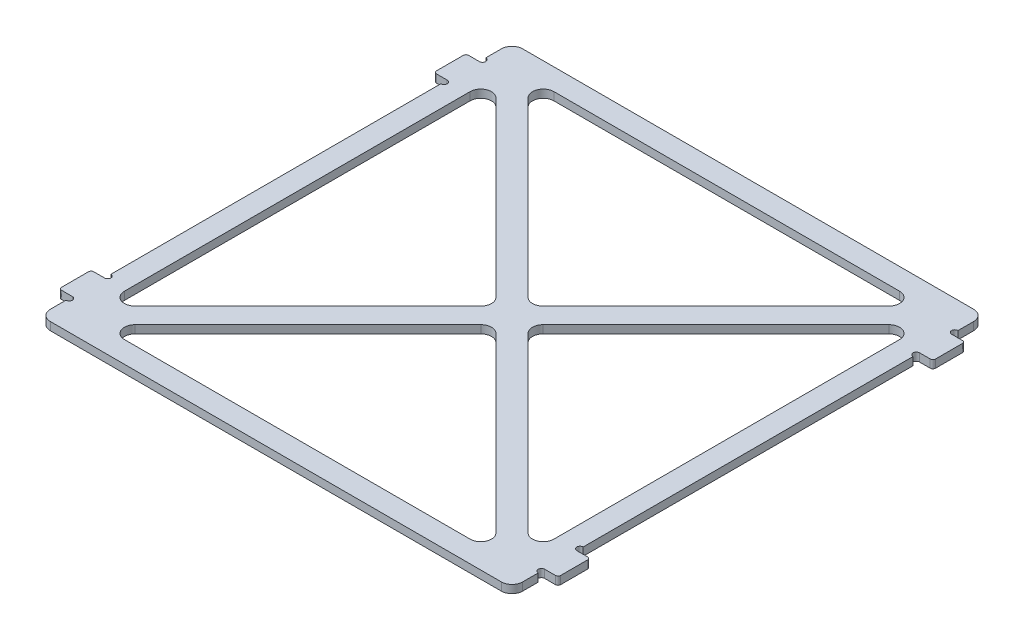
from build123d import *

# Parameters (mm, degrees)
EXTRUDE_1_DEPTH = 1.5
FILLET_1_R      = 0.5
FILLET_2_R      = 2


with BuildPart() as part:
    # 草图1 → 凸台-拉伸1 (new body)
    with BuildSketch(Plane(origin=(0, 0, 0), x_dir=(1, 0, 0), z_dir=(0, 1, 0))):
        with BuildLine():
            Line((44.1, 44.1), (-44.1, 44.1))
            Line((-44.1, 44.1), (-44.1, 39.2))
            ThreePointArc((-44.1, 39.2), (-43.5, 38.6), (-44.1, 38))
            Line((-44.1, 38), (-46.6, 38))
            Line((-46.6, 38), (-46.6, 32))
            Line((-46.6, 32), (-44.1, 32))
            ThreePointArc((-44.1, 32), (-43.5, 31.4), (-44.1, 30.8))
            Line((-44.1, 30.8), (-44.1, -30.8))
            ThreePointArc((-44.1, -30.8), (-43.5, -31.4), (-44.1, -32))
            Line((-44.1, -32), (-46.6, -32))
            Line((-46.6, -32), (-46.6, -38))
            Line((-46.6, -38), (-44.1, -38))
            ThreePointArc((-44.1, -38), (-43.5, -38.6), (-44.1, -39.2))
            Line((-44.1, -39.2), (-44.1, -44.1))
            Line((-44.1, -44.1), (44.1, -44.1))
            Line((44.1, -44.1), (44.1, -39.2))
            ThreePointArc((44.1, -39.2), (43.5, -38.6), (44.1, -38))
            Line((44.1, -38), (46.6, -38))
            Line((46.6, -38), (46.6, -32))
            Line((46.6, -32), (44.1, -32))
            ThreePointArc((44.1, -32), (43.5, -31.4), (44.1, -30.8))
            Line((44.1, -30.8), (44.1, 30.8))
            ThreePointArc((44.1, 30.8), (43.5, 31.4), (44.1, 32))
            Line((44.1, 32), (46.6, 32))
            Line((46.6, 32), (46.6, 38))
            Line((46.6, 38), (44.1, 38))
            ThreePointArc((44.1, 38), (43.5, 38.6), (44.1, 39.2))
            Line((44.1, 39.2), (44.1, 44.1))
        make_face()
        Polygon((-37.1, 40.1), (37.1, 40.1), (0, 3), align=None, mode=Mode.SUBTRACT)
        Polygon((40.1, 37.1), (40.1, -37.1), (3, 0), align=None, mode=Mode.SUBTRACT)
        Polygon((37.1, -40.1), (-37.1, -40.1), (0, -3), align=None, mode=Mode.SUBTRACT)
        Polygon((-40.1, -37.1), (-40.1, 37.1), (-3, 0), align=None, mode=Mode.SUBTRACT)
    extrude(amount=EXTRUDE_1_DEPTH)

    # 圆角1
    fillet_1_edges = [part.edges().sort_by_distance(p)[0] for p in [
        (46.6, 0.75, -38),
        (46.6, 0.75, -32),
        (46.6, 0.75, 32),
        (46.6, 0.75, 38),
        (-46.6, 0.75, 38),
        (-46.6, 0.75, 32),
        (-46.6, 0.75, -32),
        (-46.6, 0.75, -38),
    ]]
    fillet(fillet_1_edges, radius=FILLET_1_R)

    # 圆角2
    fillet_2_edges = [part.edges().sort_by_distance(p)[0] for p in [
        (-44.1, 0.75, -44.1),
        (44.1, 0.75, -44.1),
        (44.1, 0.75, 44.1),
        (-44.1, 0.75, 44.1),
        (-40.1, 0.75, 37.1),
        (-3, 0.75, 0),
        (-40.1, 0.75, -37.1),
        (37.1, 0.75, 40.1),
        (0, 0.75, 3),
        (-37.1, 0.75, 40.1),
        (3, 0.75, 0),
        (40.1, 0.75, 37.1),
        (40.1, 0.75, -37.1),
        (0, 0.75, -3),
        (37.1, 0.75, -40.1),
        (-37.1, 0.75, -40.1),
    ]]
    fillet(fillet_2_edges, radius=FILLET_2_R)


solid = part.part
